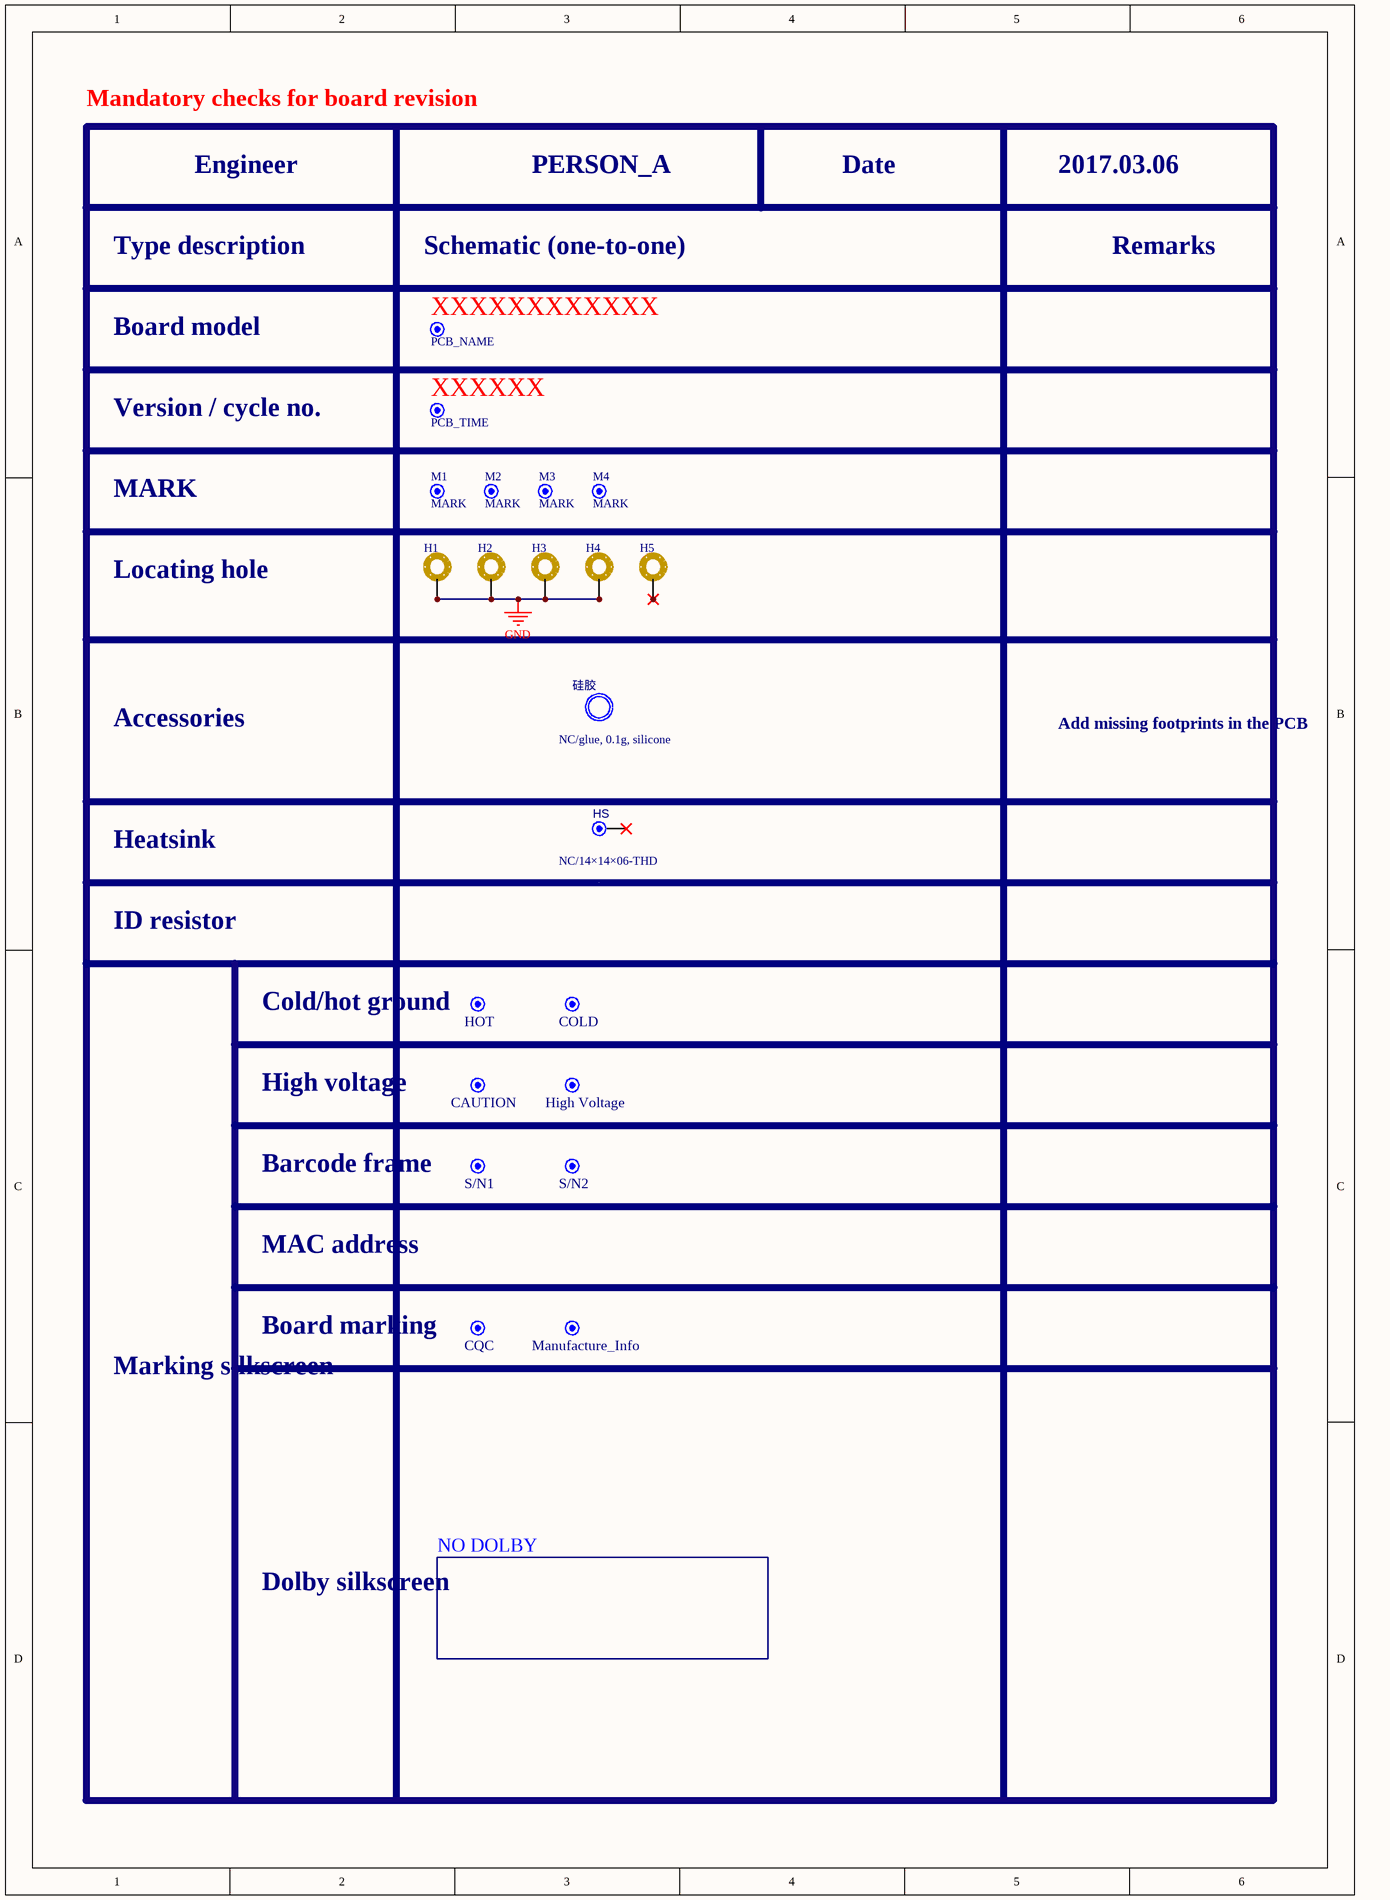
[diagram p0: MISC84277-3.SchDoc]
# Altium project MISC84277-14.PrjPCB (part 1 of 10)
9 sheets, 709 parts. Net scope: global (net labels, ports and power ports of the same name join across sheets).
Board file: MISC84277.PcbDoc
Sheets:
  MISC84277-3.SchDoc
  MISC84277-6.SchDoc
  MISC84277-7.SchDoc
  PCBE84277.SchDoc
  MISC84277-8.SchDoc
  MISC84277-9.SchDoc
  MISC84277-10.SchDoc
  MISC84277-11.SchDoc
  MISC84277-12.SchDoc

## Sheet MISC84277-3.SchDoc
size 254 x 355 mm

### Parts
CAUTION  CAUTION  [CAUTION]
COLD  COLD  [COLD]
CQC  CQC  [CQC]
H1  Location hole  [ASSE3.5C-3]  (value not drawn)
H2  Location hole  [ASSE3.5C-3]  (value not drawn)
H3  Location hole  [ASSE4.0C-4]  (value not drawn)
H4  Location hole  [ASSE5.0C-4]  (value not drawn)
H5  Location hole  [ASSE3.5C-3]  (value not drawn)
High_Voltage  High Voltage  [High Voltage]
HOT  HOT  [HOT]
HS  NC/14×14×06-THD  [HS-S]
M1  MARK  [MARK]
M2  MARK  [MARK]
M3  MARK  [MARK]
M4  MARK  [MARK]
Manufacture_Info  Manufacture_Info  [Manufacture_Info]
NO_DOLBY  NO DOLBY  [NO DOLBY-SILK]
S/N1  Barcode  [Barcode]  (value not drawn)
S/N2  Barcode  [Barcode]  (value not drawn)
XXXXXX  PCB_TIME  [PCB_TIME]
XXXXXXXXXXXX  PCB_NAME  [PCB_NAME]
硅胶  NC/glue, 0.1g, silicone  [Heat-Shrinkable Tube]

### Nets
GND: H1.0 H1.1 H1.2 H1.3 H1.4 H1.5 H1.6 H2.0 H2.1 H2.2 H2.3 H2.4 H2.5 H2.6 H3.0 H3.1 H3.2 H3.3 H3.4 H3.5 H3.6 H4.0 H4.1 H4.2 H4.3 H4.4 H4.5 H4.6
NetH5_0: H5.0 H5.1 H5.2 H5.3 H5.4 H5.5 H5.6

Not connected (* = marked no-connect by the designer): HS 1*

### Notes on the sheet
- Mandatory checks for board revision
- Engineer
- PERSON_A
- Date
- 2017.03.06
- Type description
- Schematic (one-to-one)
- Remarks
- Board model
- Version / cycle no.
- MARK
- Locating hole
- Accessories
- Add missing footprints in the PCB
- Heatsink
- ID resistor
- (near HOT) Cold/hot ground
- High voltage
- (near S/N1) Barcode frame
- MAC address
- Marking silkscreen
- (near CQC) Board marking
- (near NO_DOLBY) Dolby silkscreen

### Library data of the parts
H1-H5 = Location hole-D
HS = TEST
M1-M4 = MARK-D
硅胶 = Φ12mm×12mm-黑色-125度(UL认证)-D